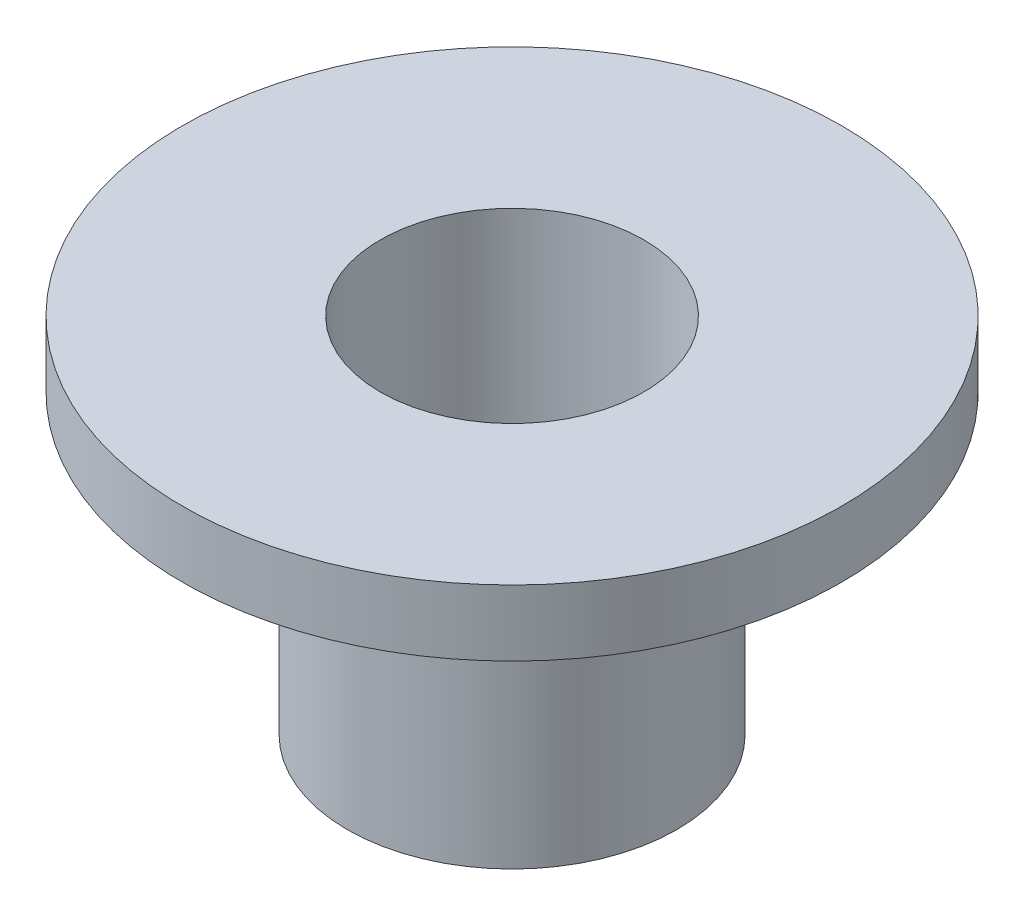
from build123d import *


with BuildPart() as part:
    # Sketch1 → Revolve1 (revolve)
    with BuildSketch(Plane.XY, mode=Mode.PRIVATE) as revolve1_sk:
        Polygon((2, 5.5), (5, 5.5), (5, 4.5), (2.5, 4.5), (2.5, 0), (2, 0), align=None)
    revolve(revolve1_sk.sketch.rotate(Axis((0, 0, 0), (0, 1, 0)), 90), axis=Axis((0, 0, 0), (0, 1, 0)))


solid = part.part
